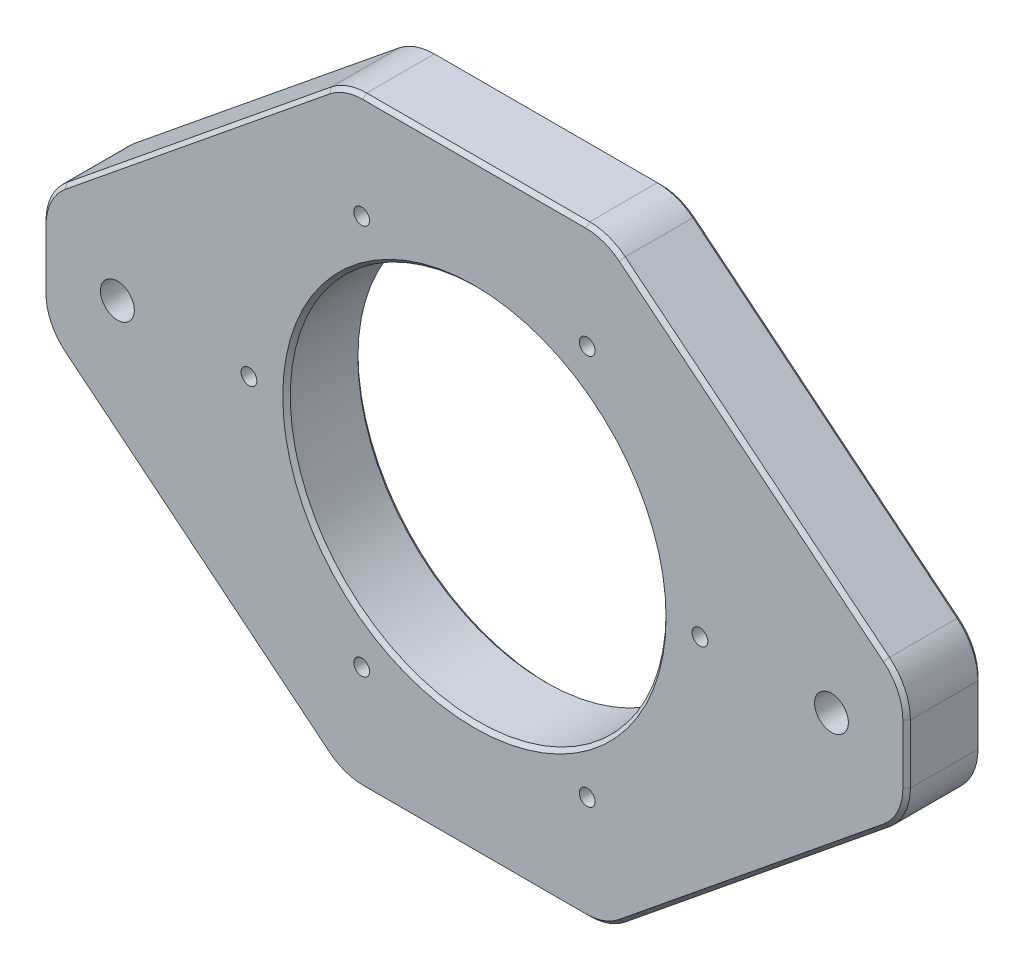
from build123d import *

# Parameters (mm, degrees)
SKETCH1_W            = 230
SKETCH1_H            = 160
BOSS_EXTRUDE1_DEPTH  = 20
SKETCH4_R            = 50
CUT_EXTRUDE3_DEPTH   = 109
SKETCH5_R            = 10.25
CUT_EXTRUDE4_DEPTH   = 6
M8_CLEARANCE_HOLE1_D = 9
CHAMFER2_SIZE        = 1
CUT_EXTRUDE6_DEPTH   = 214
FILLET1_R            = 15
CHAMFER3_SIZE        = 1
CHAMFER4_SIZE        = 1
M5_TAPPED_HOLE1_D    = 4.2


with BuildPart() as part:
    # Sketch1 → Boss-Extrude1 (new body)
    with BuildSketch(Plane.XY):
        Rectangle(SKETCH1_W, SKETCH1_H)
    extrude(amount=BOSS_EXTRUDE1_DEPTH)

    # Sketch4 → Cut-Extrude3 (cut)
    with BuildSketch(Plane.XY.offset(20)):
        Circle(SKETCH4_R)
    extrude(amount=-CUT_EXTRUDE3_DEPTH, mode=Mode.SUBTRACT)

    # Sketch5 → Cut-Extrude4 (cut)
    with BuildSketch(Plane.XY):
        with Locations((-95, 0)):
            Circle(SKETCH5_R)
        with Locations((95, 0)):
            Circle(SKETCH5_R)
    extrude(amount=CUT_EXTRUDE4_DEPTH, mode=Mode.SUBTRACT)

    # M8 Clearance Hole1 (through all)
    with Locations(Plane.XY.offset(20)):
        with Locations((-95, 0), (95, 0)):
            Hole(M8_CLEARANCE_HOLE1_D / 2)

    # Chamfer2
    chamfer2_edges = [part.edges().sort_by_distance(p)[0] for p in [
        (-50, 0, 0),
        (-50, 0, 20),
    ]]
    chamfer(chamfer2_edges, length=CHAMFER2_SIZE)

    # Sketch10 → Cut-Extrude6 (cut)
    with BuildSketch(Plane.XY.offset(20)):
        Polygon((-115, 80), (-35, 80), (-115, 15), align=None)
        Polygon((35, 80), (115, 80), (115, 15), align=None)
        Polygon((-115, -15), (-35, -80), (-115, -80), align=None)
        Polygon((35, -80), (115, -80), (115, -15), align=None)
    extrude(amount=-CUT_EXTRUDE6_DEPTH, mode=Mode.SUBTRACT)

    # Fillet1
    fillet1_edges = [part.edges().sort_by_distance(p)[0] for p in [
        (115, 15, 10),
        (35, 80, 10),
        (-115, -15, 10),
        (-35, -80, 10),
        (35, -80, 10),
        (115, -15, 10),
        (-115, 15, 10),
        (-35, 80, 10),
    ]]
    fillet(fillet1_edges, radius=FILLET1_R)

    # Chamfer3
    chamfer3_edges = [part.edges().sort_by_distance(p)[0] for p in [
        (-74.296084687, 48.071931192, 0),
        (-74.296084687, 48.071931192, 20),
        (115, 0, 20),
        (74.296084687, 48.071931192, 20),
        (0, 80, 20),
        (-115, 0, 20),
        (-74.296084687, -48.071931192, 20),
        (0, -80, 20),
        (74.296084687, -48.071931192, 20),
        (-113.544064025, -14.307017415, 20),
        (-34.693073216, -79.13551644, 20),
        (34.693073216, -79.13551644, 20),
        (113.544064025, -14.307017415, 20),
        (113.544064025, 14.307017415, 20),
        (34.693073216, 79.13551644, 20),
        (-34.693073216, 79.13551644, 20),
        (-113.544064025, 14.307017415, 20),
        (-115, 0, 0),
        (74.296084687, 48.071931192, 0),
        (115, 0, 0),
        (74.296084687, -48.071931192, 0),
        (0, -80, 0),
        (-74.296084687, -48.071931192, 0),
        (0, 80, 0),
        (-113.544064025, -14.307017415, 0),
        (-34.693073216, -79.13551644, 0),
        (34.693073216, -79.13551644, 0),
        (113.544064025, -14.307017415, 0),
        (113.544064025, 14.307017415, 0),
        (34.693073216, 79.13551644, 0),
        (-34.693073216, 79.13551644, 0),
        (-113.544064025, 14.307017415, 0),
    ]]
    chamfer(chamfer3_edges, length=CHAMFER3_SIZE)

    # Chamfer4
    chamfer4_edges = [part.edges().sort_by_distance(p)[0] for p in [
        (-105.25, 0, 0),
        (84.75, 0, 0),
    ]]
    chamfer(chamfer4_edges, length=CHAMFER4_SIZE)

    # M5 Tapped Hole1 (through all)
    with Locations(Plane.XY.offset(20)):
        with Locations((-30, 51.961524227), (-60, 0), (-30, -51.961524227), (30, -51.961524227), (60, 0), (30, 51.961524227)):
            Hole(M5_TAPPED_HOLE1_D / 2)


solid = part.part
